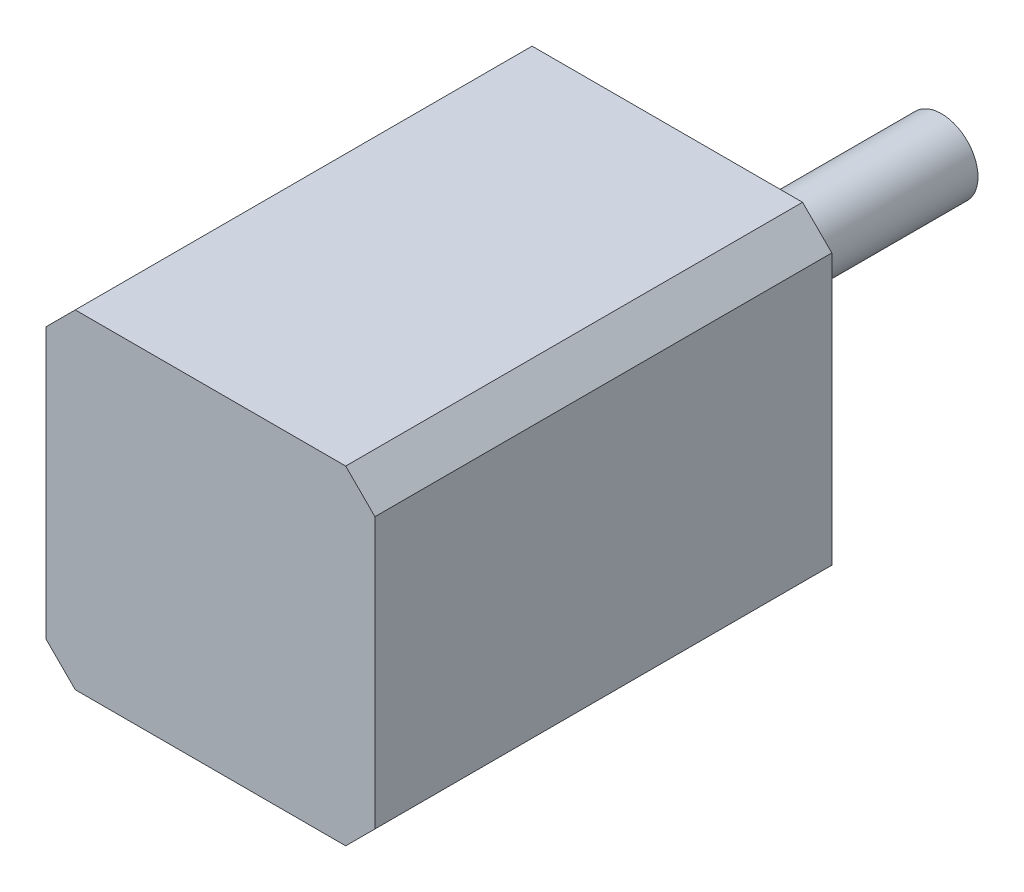
SolidWorks part; units mm, degrees
ref_plane "Front Plane" through (0, 0, 0) normal (0, 0, 1) x (1, 0, 0)
ref_plane "Top Plane" through (0, 0, 0) normal (0, 1, 0) x (1, 0, 0)
ref_plane "Right Plane" through (0, 0, 0) normal (1, 0, 0) x (0, 0, -1)
sketch "Sketch1" plane through (0, 0, 0) normal (0, 0, 1) x (1, 0, 0)
  circle A0 centre (0, 0) radius 20
  dimension "D1" = 40
extrude "Boss-Extrude1" add sketch "Sketch1" along normal blind 140
sketch "Sketch2" plane through (0, 0, 140) normal (0, 0, 1) x (1, 0, 0)
  circle A0 centre (0, 0) radius 45
  dimension "D1" = 90
extrude "Boss-Extrude2" add sketch "Sketch2" along normal blind 10
sketch "Sketch3" plane through (0, 0, 150) normal (0, 0, 1) x (1, 0, 0)
  line L1 (-90, 90) -> (90, 90)
  line L2 (-90, 90) -> (-90, -90)
  line L3 (-90, -90) -> (90, -90)
  line L4 (90, 90) -> (90, -90)
  line L5 (-90, 90) -> (90, -90) construction
  line L6 (-90, -90) -> (90, 90) construction
  point P0 (0, 0)
  dimension "D1" = 180
  dimension "D2" = 180
extrude "Boss-Extrude3" add sketch "Sketch3" along normal blind 250
chamfer "Chamfer1" distance 16 angle 45 4 edges at (90, -90, 275) (-90, -90, 275) (-90, 90, 275) (90, 90, 275)
